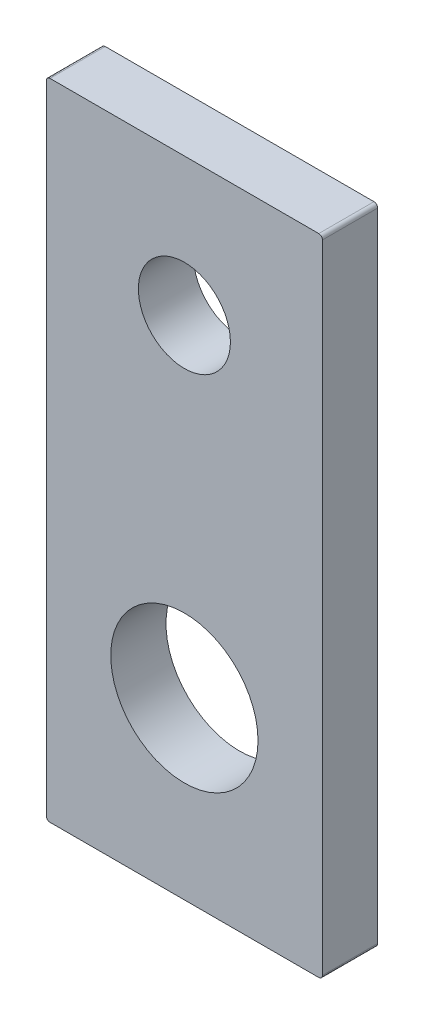
from build123d import *

# Parameters (mm, degrees)
SKETCH1_W           = 150
SKETCH1_H           = 350
BOSS_EXTRUDE1_DEPTH = 30
SKETCH2_R           = 25
SKETCH2_R_2         = 40
CUT_EXTRUDE1_DEPTH  = 30
FILLET1_R           = 2


with BuildPart() as part:
    # Sketch1 → Boss-Extrude1 (new body)
    with BuildSketch(Plane.XY):
        Rectangle(SKETCH1_W, SKETCH1_H)
    extrude(amount=BOSS_EXTRUDE1_DEPTH)

    # Sketch2 → Cut-Extrude1 (cut)
    with BuildSketch(Plane.XY.offset(30)):
        with Locations((0, 100)):
            Circle(SKETCH2_R)
        with Locations((0, -80)):
            Circle(SKETCH2_R_2)
    extrude(amount=-CUT_EXTRUDE1_DEPTH, mode=Mode.SUBTRACT)

    # Fillet1
    fillet1_edges = [part.edges().sort_by_distance(p)[0] for p in [
        (-75, 175, 15),
        (75, 175, 15),
        (75, -175, 15),
        (-75, -175, 15),
    ]]
    fillet(fillet1_edges, radius=FILLET1_R)


solid = part.part
